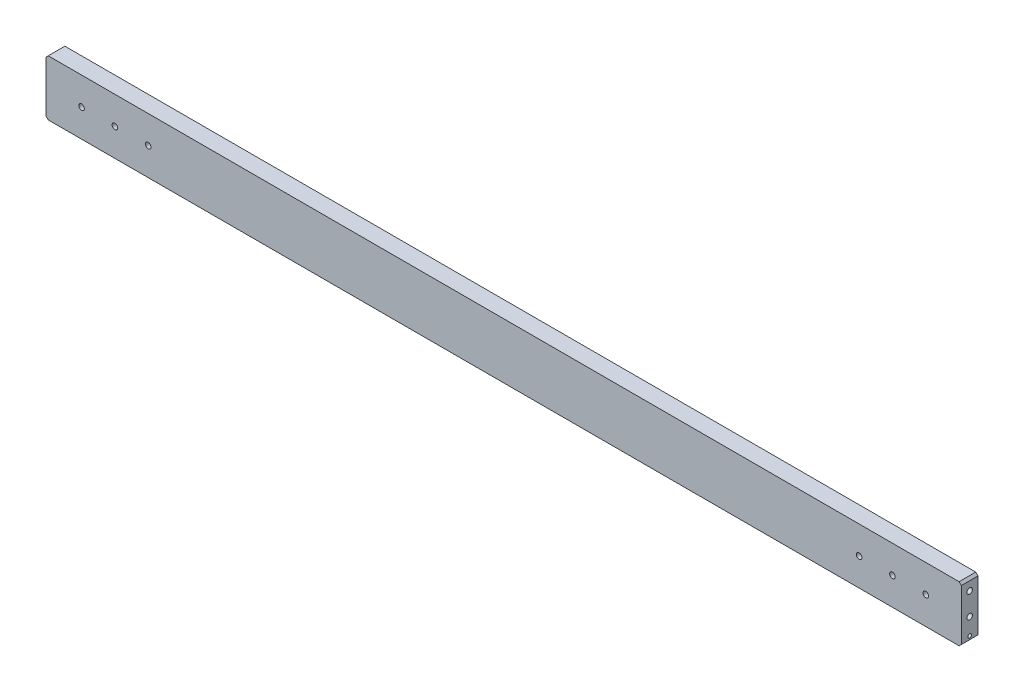
from build123d import *

# Parameters (mm, degrees)
SKETCH_1_W                  = 824
SKETCH_1_H                  = 50
EXTRUDE_1_DEPTH             = 15
HOLE_WIZARD_M6_1_AT_2_COUNT = 2
HOLE_WIZARD_M6_1_AT_2_PITCH = 19.9999375
HOLE_WIZARD_M6_2_D          = 5
HOLE_WIZARD_M6_2_DEPTH      = 17
HOLE_WIZARD_M6_2_TIP        = 1.502151548
CHAMFER_1_SIZE              = 2


with BuildPart() as part:
    # 草图1 → 凸台-拉伸1 (new body)
    with BuildSketch(Plane.XY):
        with Locations((-412, 25)):
            Rectangle(SKETCH_1_W, SKETCH_1_H)
    extrude(amount=EXTRUDE_1_DEPTH)

    # 草图3 → M6 螺纹孔1 (revolve, cut)
    with BuildSketch(Plane(origin=(0, 40, 7.5), x_dir=(0, 0, -1), z_dir=(0, 1, 0))):
        Polygon((0, 0), (0, 18.502151548), (2.5, 17), (2.5, 0), align=None)
    hole_wizard_m6_1 = revolve(axis=Axis((6.35, 40, 7.5), (-1, 0, 0)), mode=Mode.SUBTRACT)

    # M6 螺纹孔1 at 2: M6 螺纹孔1 ×2
    with Locations(*[(0, -i * HOLE_WIZARD_M6_1_AT_2_PITCH, 0) for i in range(1, HOLE_WIZARD_M6_1_AT_2_COUNT)]):
        add(hole_wizard_m6_1, mode=Mode.SUBTRACT)

    # 草图5 → M4 螺纹孔1 (revolve, cut)
    with BuildSketch(Plane(origin=(0, 5.000249994, 7.5), x_dir=(0, 0, -1), z_dir=(0, 1, 0))):
        Polygon((0, 0), (0, 12.491420021), (1.65, 11.5), (1.65, 0), align=None)
    hole_wizard_m4_1 = revolve(axis=Axis((6.35, 5.000249994, 7.5), (-1, 0, 0)), mode=Mode.SUBTRACT)

    # 镜向1: M6 螺纹孔1, M4 螺纹孔1 across plane
    add(hole_wizard_m6_1.mirror(Plane(origin=(-412, 0, 0), x_dir=(0, 0, 1), z_dir=(1, 0, 0))), mode=Mode.SUBTRACT)
    add(hole_wizard_m4_1.mirror(Plane(origin=(-412, 0, 0), x_dir=(0, 0, 1), z_dir=(1, 0, 0))), mode=Mode.SUBTRACT)

    # 镜向1 copy 1 sketch → 镜向1 copy 1 (revolve, cut)
    with BuildSketch(Plane(origin=(-824, 20.0000625, 7.5), x_dir=(0, 0, -1), z_dir=(0, 1, 0))):
        Polygon((0, 0), (0, -18.502151548), (2.5, -17), (2.5, 0), align=None)
    revolve(axis=Axis((-830.35, 20.0000625, 7.5), (-1, 0, 0)), mode=Mode.SUBTRACT)

    # M6 螺纹孔2
    with Locations(Plane(origin=(0, 0, 0), x_dir=(-1, 0, 0), z_dir=(0, 0, -1))):
        with Locations((792, 25), (32, 25), (62, 25), (92, 25), (732, 25), (762, 25)):
            Hole(HOLE_WIZARD_M6_2_D / 2, depth=HOLE_WIZARD_M6_2_DEPTH)
            with Locations((0, 0, -(HOLE_WIZARD_M6_2_DEPTH + HOLE_WIZARD_M6_2_TIP / 2))):  # 118° drill point
                Cone(0, HOLE_WIZARD_M6_2_D / 2, HOLE_WIZARD_M6_2_TIP, mode=Mode.SUBTRACT)

    # 倒角1
    chamfer_1_edges = [part.edges().sort_by_distance(p)[0] for p in [
        (0, 50, 7.5),
        (0, 0, 7.5),
        (-824, 0, 7.5),
        (-824, 50, 7.5),
    ]]
    chamfer(chamfer_1_edges, length=CHAMFER_1_SIZE)


solid = part.part
